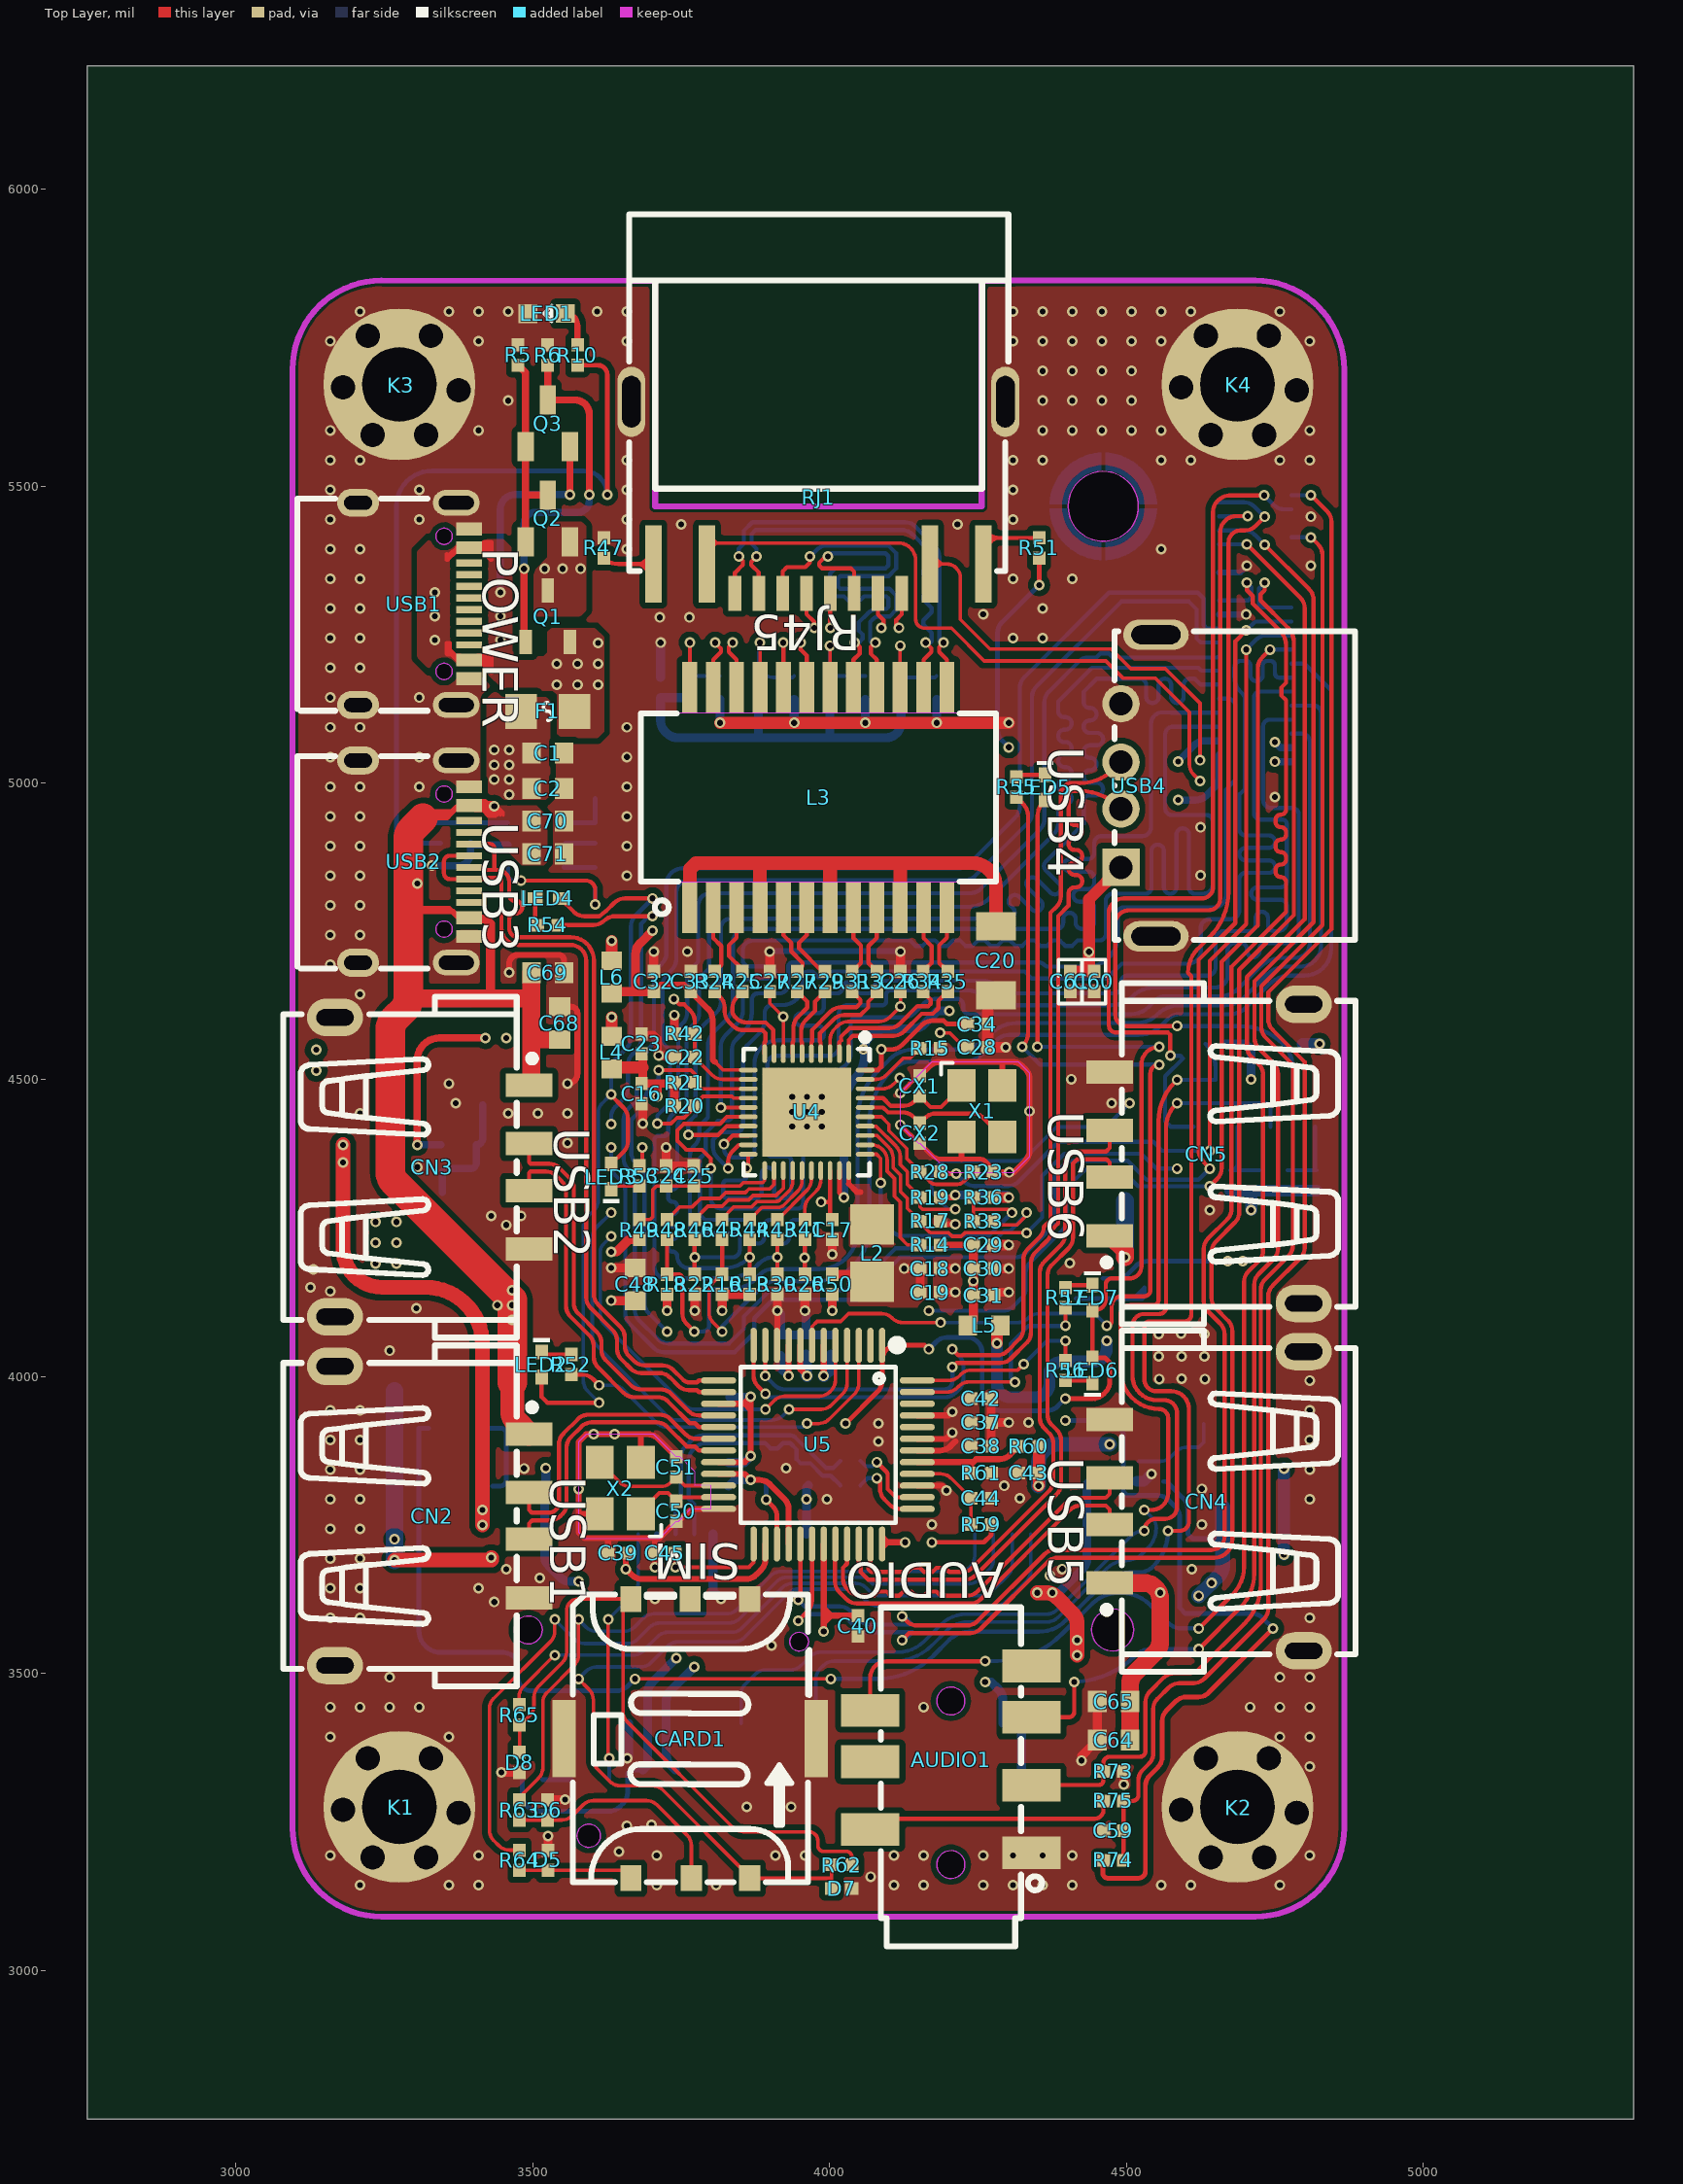
[diagram p0: Top Layer view]
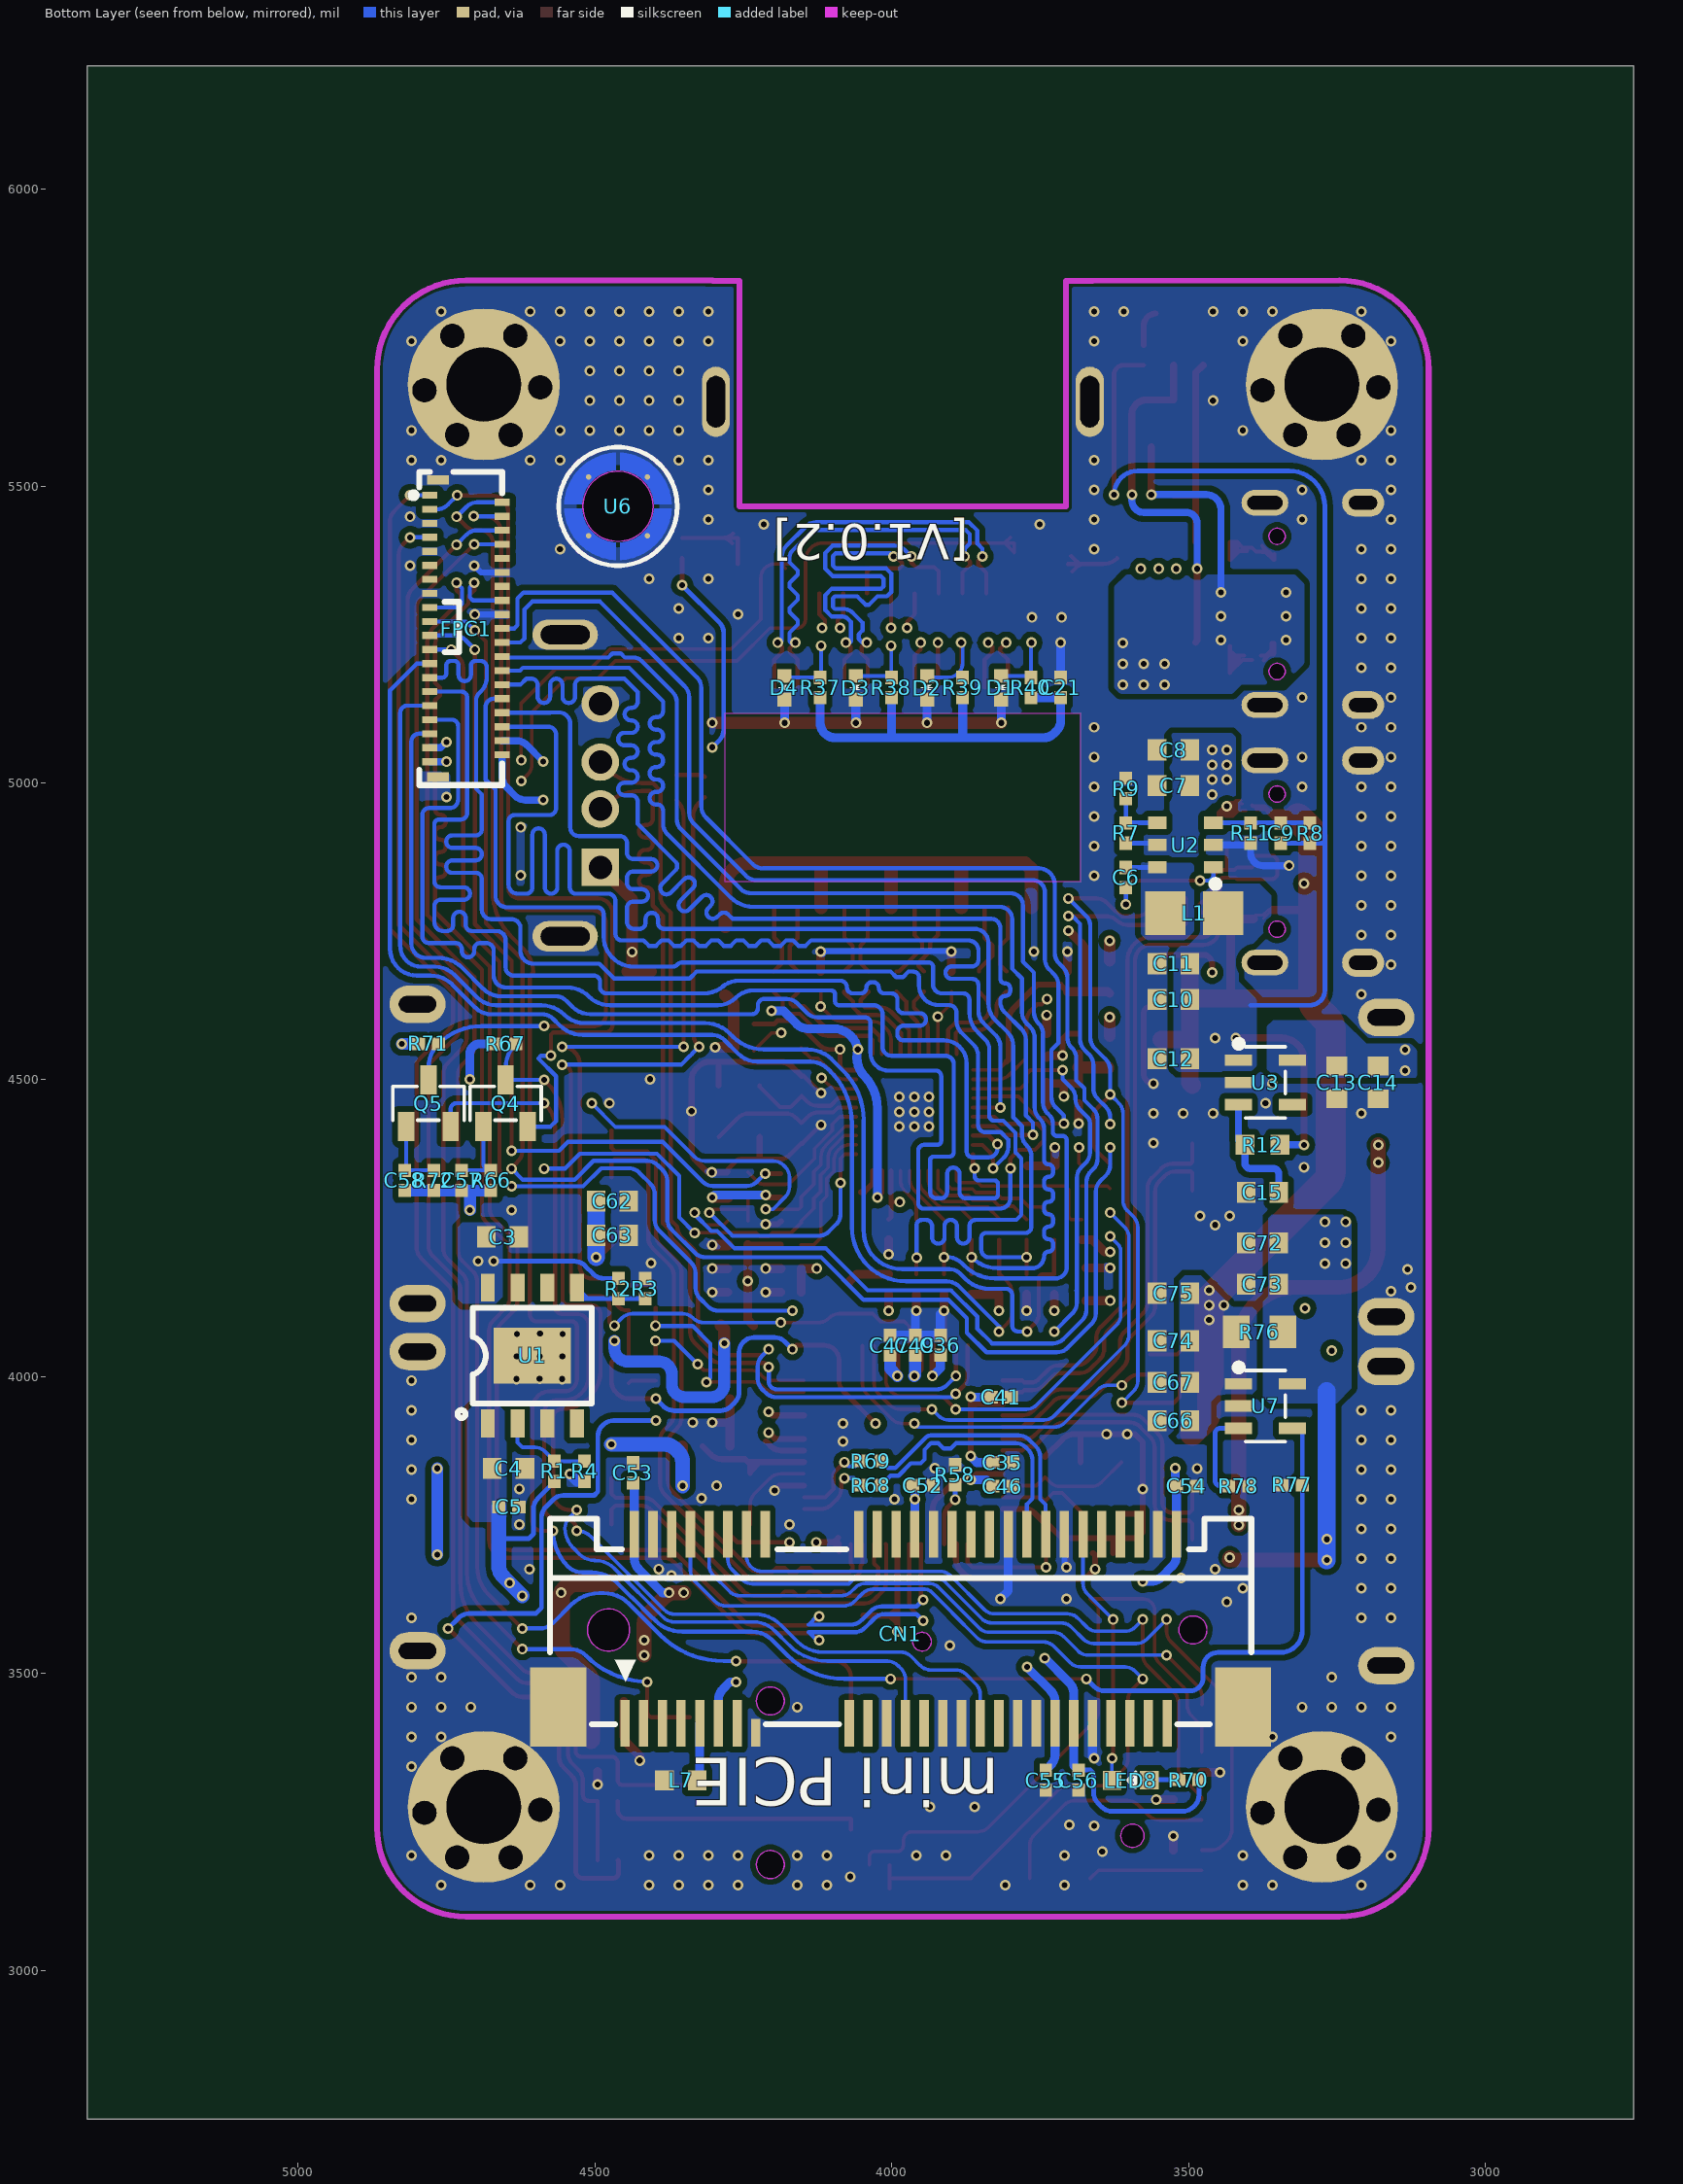
[diagram p1: Bottom Layer view, seen from below]
# Altium PCB MISC84334.PcbDoc (part 1 of 8)
Units mil, origin at the board's own origin, x right, y up, seen from the top; angles counter-clockwise.
Board outline 2605.13 x 3457.4 mil, 4 copper layers (Top Layer, GND, VCC, Bottom Layer), stack 62.447 mil thick; 209 components, 149 nets, 735 pads, 529 vias.

## Layer stack, top to bottom
Top Layer: signal copper 1.378
Dielectric1: surface 8.283, 7628 RC49% 8.6mil, Dk 0
GND: signal copper 0.598
Dielectric2: surface 41.929, 1.1mm H/HOZ 含铜, Dk 0
VCC: signal copper 0.598
Dielectric3: surface 8.283, 7628 RC49% 8.6mil, Dk 0
Bottom Layer: signal copper 1.378

## Board outline
5355.13,2750 2750,2750 2750,6207.4 5355.13,6207.4

## Design rules (kind name [scope] priority, off if disabled: settings)
BoardOutlineClearance copperThickness2oz_1 [All] p2 off: genericclearance=8 ignorepadtopadclearanceinfootprint=FALSE except(0: Arc-SplitContinuation Track-SplitContinuation SMDPad-SplitContinuation THPad-SplitContinuation Via-SplitContinuation Fill-SplitContinuation Region-SplitContinuation Poly-SplitContinuation Text-SplitContinuation Hole-SplitContinuation; 6: Arc-OutlineEdge Track-OutlineEdge SMDPad-OutlineEdge THPad-OutlineEdge Via-OutlineEdge Fill-OutlineEdge Region-OutlineEdge Text-OutlineEdge Hole-OutlineEdge Arc-CutoutEdge Track-CutoutEdge SMDPad-CutoutEdge THPad-CutoutEdge Via-CutoutEdge Fill-CutoutEdge Region-CutoutEdge Text-CutoutEdge Hole-CutoutEdge; 10: Poly-OutlineEdge Poly-CutoutEdge)
BoardOutlineClearance Plane_innerPlane_1 [All] p4 off: genericclearance=4 ignorepadtopadclearanceinfootprint=FALSE except(0: SMDPad-CutoutEdge Arc-SplitContinuation Track-SplitContinuation SMDPad-SplitContinuation THPad-SplitContinuation Via-SplitContinuation Fill-SplitContinuation Region-SplitContinuation Poly-SplitContinuation Text-SplitContinuation Hole-SplitContinuation; 6: Arc-OutlineEdge Track-OutlineEdge SMDPad-OutlineEdge THPad-OutlineEdge Via-OutlineEdge Fill-OutlineEdge Region-OutlineEdge Text-OutlineEdge Hole-OutlineEdge Arc-CutoutEdge Track-CutoutEdge THPad-CutoutEdge Via-CutoutEdge Fill-CutoutEdge Region-CutoutEdge Text-CutoutEdge Hole-CutoutEdge; 10: Poly-OutlineEdge Poly-CutoutEdge)
BoardOutlineClearance Copper_copperRegion_1 [All] p6 off: genericclearance=4 ignorepadtopadclearanceinfootprint=FALSE except(0: SMDPad-CutoutEdge Arc-SplitContinuation Track-SplitContinuation SMDPad-SplitContinuation THPad-SplitContinuation Via-SplitContinuation Fill-SplitContinuation Region-SplitContinuation Poly-SplitContinuation Text-SplitContinuation Hole-SplitContinuation; 6: Arc-OutlineEdge Track-OutlineEdge SMDPad-OutlineEdge THPad-OutlineEdge Via-OutlineEdge Fill-OutlineEdge Region-OutlineEdge Text-OutlineEdge Hole-OutlineEdge Arc-CutoutEdge Track-CutoutEdge THPad-CutoutEdge Via-CutoutEdge Fill-CutoutEdge Region-CutoutEdge Text-CutoutEdge Hole-CutoutEdge; 10: Poly-OutlineEdge Poly-CutoutEdge)
BoardOutlineClearance copperThickness1oz_1 [All] p8: genericclearance=4 ignorepadtopadclearanceinfootprint=FALSE except(0: SMDPad-CutoutEdge Arc-SplitContinuation Track-SplitContinuation SMDPad-SplitContinuation THPad-SplitContinuation Via-SplitContinuation Fill-SplitContinuation Region-SplitContinuation Poly-SplitContinuation Text-SplitContinuation Hole-SplitContinuation; 6: Arc-OutlineEdge Track-OutlineEdge SMDPad-OutlineEdge THPad-OutlineEdge Via-OutlineEdge Fill-OutlineEdge Region-OutlineEdge Text-OutlineEdge Hole-OutlineEdge Arc-CutoutEdge Track-CutoutEdge THPad-CutoutEdge Via-CutoutEdge Fill-CutoutEdge Region-CutoutEdge Text-CutoutEdge Hole-CutoutEdge; 10: Poly-OutlineEdge Poly-CutoutEdge)
Clearance copperThickness2oz [All] p1 off: gap=8 ignorepadtopadclearanceinfootprint=FALSE except(6: SMDPad-Track SMDPad-SMDPad THPad-Track SMDPad-THPad THPad-THPad Track-Via SMDPad-Via THPad-Via Via-Via Fill-Track Region-Track Fill-SMDPad Region-SMDPad Fill-THPad Region-THPad Fill-Via Region-Via Fill-Fill Fill-Region Region-Region Arc-SMDPad Arc-THPad Arc-Via Fill-Arc Region-Arc Arc-Arc Text-Track SMDPad-Text Text-THPad Text-Via Fill-Text Region-Text Text-Text Hole-Track Hole-SMDPad Hole-THPad Hole-Via Fill-Hole Region-Hole Hole-Arc Hole-Text; 10: Poly-Track Poly-SMDPad Poly-THPad Poly-Via Poly-Fill Poly-Region Poly-Poly Poly-Arc Poly-Text Poly-Hole; 11.8: Arc-Track Arc-Text)
Clearance Plane_innerPlane [All] p3 off: gap=4 ignorepadtopadclearanceinfootprint=FALSE except(6: SMDPad-Track SMDPad-SMDPad THPad-Track SMDPad-THPad THPad-THPad Track-Via SMDPad-Via THPad-Via Via-Via Fill-Track Region-Track Fill-SMDPad Region-SMDPad Fill-THPad Region-THPad Fill-Via Region-Via Fill-Fill Fill-Region Region-Region Arc-SMDPad Arc-THPad Arc-Via Fill-Arc Region-Arc Arc-Arc Text-Track SMDPad-Text Text-THPad Text-Via Fill-Text Region-Text Text-Text Hole-Track Hole-SMDPad Hole-THPad Hole-Via Fill-Hole Region-Hole Hole-Arc Hole-Text; 10: Poly-Track Poly-SMDPad Poly-THPad Poly-Via Poly-Fill Poly-Region Poly-Poly Poly-Arc Poly-Text Poly-Hole; 11.8: Arc-Track Arc-Text)
Clearance Copper_copperRegion [All] p5 off: gap=4 ignorepadtopadclearanceinfootprint=FALSE except(6: SMDPad-Track SMDPad-SMDPad THPad-Track SMDPad-THPad THPad-THPad Track-Via SMDPad-Via THPad-Via Via-Via Fill-Track Region-Track Fill-SMDPad Region-SMDPad Fill-THPad Region-THPad Fill-Via Region-Via Fill-Fill Fill-Region Region-Region Arc-SMDPad Arc-THPad Arc-Via Fill-Arc Region-Arc Arc-Arc Text-Track SMDPad-Text Text-THPad Text-Via Fill-Text Region-Text Text-Text Hole-Track Hole-SMDPad Hole-THPad Hole-Via Fill-Hole Region-Hole Hole-Arc Hole-Text; 10: Poly-Track Poly-SMDPad Poly-THPad Poly-Via Poly-Fill Poly-Region Poly-Poly Poly-Arc Poly-Text Poly-Hole; 11.8: Arc-Track Arc-Text)
Clearance copperThickness1oz [All] p7: gap=4 ignorepadtopadclearanceinfootprint=FALSE except(6: SMDPad-Track SMDPad-SMDPad THPad-Track SMDPad-THPad THPad-THPad Track-Via SMDPad-Via THPad-Via Via-Via Fill-Track Region-Track Fill-SMDPad Region-SMDPad Fill-THPad Region-THPad Fill-Via Region-Via Fill-Fill Fill-Region Region-Region Arc-SMDPad Arc-THPad Arc-Via Fill-Arc Region-Arc Arc-Arc Text-Track SMDPad-Text Text-THPad Text-Via Fill-Text Region-Text Text-Text Hole-Track Hole-SMDPad Hole-THPad Hole-Via Fill-Hole Region-Hole Hole-Arc Hole-Text; 10: Poly-Track Poly-SMDPad Poly-THPad Poly-Via Poly-Fill Poly-Region Poly-Poly Poly-Arc Poly-Text Poly-Hole; 11.8: Arc-Track Arc-Text)
DiffPairsRouting differentialPair [All] p1: maxlimit=6 minlimit=6 mostfreqgap=6 toplayer_minwidth=7 toplayer_prefwidth=7 toplayer_maxwidth=7 toplayer_mingap=6 toplayer_prefgap=6 toplayer_maxgap=6 midlayer1_minwidth=7 midlayer1_prefwidth=7 midlayer1_maxwidth=7 midlayer1_mingap=6 midlayer1_prefgap=6 midlayer1_maxgap=6 midlayer2_minwidth=7 midlayer2_prefwidth=7 midlayer2_maxwidth=7 midlayer2_mingap=6 midlayer2_prefgap=6 midlayer2_maxgap=6 bottomlayer_minwidth=7 bottomlayer_prefwidth=7 bottomlayer_maxwidth=7 bottomlayer_mingap=6 bottomlayer_prefgap=6 bottomlayer_maxgap=6 maxuncoupledlength=10
HoleToHoleClearance otherClearance [All] p1: gap=11.8 allowstackedmicrovias=TRUE
Length netLength [All] p1: minlimit=0 maxlimit=0
PasteMaskExpansion pasteMaskExpansion [All] p1: expansion=0
PlaneConnect innerPlane [All] p1: planeconnectstyle=Relief reliefexpansion=20 reliefentries=4 reliefconductorwidth=10 reliefairgap=10
PolygonConnect copperRegion [All] p1: connectstyle=Direct reliefconductorwidth=10 reliefentries=4 polygonreliefangle="90 Angle" airgapwidth=10 via.connectstyle=Relief via.reliefconductorwidth=10 via.reliefentries=4 via.polygonreliefangle="90 Angle" via.airgapwidth=10
RoutingVias viaSize [All] p1: holewidth=10 width=18 viastyle="Through Hole" minholewidth=10 minwidth=18 maxholewidth=10 maxwidth=18
SolderMaskExpansion solderMaskExpansion [IsVia] p1: expansion=-1000 istentingtop=TRUE
SolderMaskExpansion solderMaskExpansion [All] p2: expansion=2 istentingtop=FALSE
Width copperThickness2oz_2 [All] p1 off: maxlimit=100 minlimit=8 preferedwidth=10
Width copperThickness1oz_2 [All] p2: maxlimit=100 minlimit=5 preferedwidth=7

## Components (designator, comment, footprint, x,y, rotation, side; value= is the part's Value field where it differs from the comment)
AUDIO1 "PJ-393" AUDIO-SMD_PJ-393 4204.62,3355.59 r0 top
C1 "10uF" r0603#1 3525.59,5050.59 r180 top
C2 "100nF" r0603#1 3525.59,4990.59 r180 top
C3 "4.7uF" C0603 4655.59,4235.59 r0 bottom
C4 "4.7uF" C0603 4645.59,3845.59 r0 bottom
C5 "100nF" R0402 4645.29,3780.59 r0 bottom
C6 "100nF" R0402 3605.59,4840.59 r270 bottom
C7 "10uF" r0603#2 3525.59,4995.59 r180 bottom
C8 "100nF" r0603#2 3525.59,5055.59 r180 bottom
C9 "22pF" R0402 3344.86,4915.59 r270 bottom
C10 "22uF" r0603#2 3525.59,4635.59 r180 bottom
C11 "100nF" r0603#2 3525.59,4695.59 r180 bottom
C12 "10uF" r0603#1 3525.59,4535.59 r180 bottom
C13 "4.7uF" r0603#1 3250.59,4495.59 r90 bottom
C14 "100nF" C0603 3180.59,4495.59 r90 bottom
C15 "100nF" C0603 3375.59,4310.59 r180 bottom
C16 "100nF" R0402 3683.59,4476.71 r90 top
C17 "100nF" R0402 4005.09,4247.85 r90 top
C18 "100nF" R0402 4169.59,4182.09 r180 top
C19 "4.7uF" R0402 4169.83,4142.09 r180 top
C20 "10nF" r1206 4280.59,4700.59 r90 top
C21 "1nF" R0402 3715.59,5160.59 r270 bottom
C22 "100nF" R0402 3756.09,4538.09 r0 top
C23 "100nF" R0402 3683.59,4560.59 r270 top
C24 "100nF" R0402 3725.09,4338.09 r270 top
C25 "100nF" R0402 3771.52,4338.09 r270 top
C26 "100nF" R0402 4119.79,4665.59 r270 top
C27 "100nF" R0402 3899.65,4665.59 r270 top
C28 "100nF" R0402 4249.48,4555.09 r180 top
C29 "100nF" R0402 4259.59,4222.09 r180 top
C30 "100nF" R0402 4259.59,4182.09 r180 top
C31 "100nF" R0402 4259.59,4137.09 r180 top
C32 "100nF" R0402 3704.09,4665.59 r270 top
C33 "100nF" R0402 3766.55,4665.59 r270 top
C34 "100nF" R0402 4249.48,4594.09 r180 top
C35 "100nF" R0402 3813.09,3855.59 r0 bottom
C36 "100nF" R0402 3918.09,4053.09 r270 bottom
C37 "100nF" R0402 4255.6,3923.09 r180 top
C38 "100nF" R0402 4255.6,3883.09 r180 top
C39 "100nF" R0402 3644.19,3703.09 r0 top
C40 "100nF" R0402 4048.09,3580.59 r90 top
C41 "100nF" R0402 3815.59,3965.59 r0 bottom
C42 "100nF" R0402 4255.6,3963.09 r180 top
C43 "100nF" R0402 4335.95,3838.09 r0 top
C44 "100nF" R0402 4255.6,3795.59 r180 top
C45 "100nF" R0402 3723.14,3703.09 r0 top
C46 "100nF" R0402 3813.09,3815.59 r0 bottom
C47 "100nF" R0402 4003.09,4053.09 r270 bottom
C48 "10uF" r0603#1 3673,4155.59 r270 top
C49 "100nF" R0402 3960.59,4053.09 r270 bottom
C50 "12pF" R0402 3742.02,3773.39 r90 top
C51 "12pF" R0402 3742.02,3848.09 r90 top
C52 "100nF" R0402 3947.55,3817.03 r0 bottom
C53 "100nF" R0402 4436.02,3838.07 r270 bottom
C54 "100nF" R0402 3503.47,3816.03 r0 bottom
C55 "100nF" R0402 3740.59,3320.59 r90 bottom
C56 "100nF" R0402 3685.59,3320.59 r90 bottom
C57 "1nF" r0402 4724.41,4330.59 r90 bottom
C58 "1nF" r0402 4820.59,4330.59 r270 bottom
C59 "100nF" R0402 4478.65,3235.59 r180 top
C60 "100nF" R0402 4445.59,4665.59 r90 top
C61 "10uF" R0402 4405.59,4665.59 r90 top
C62 "100nF" r0603#1 4470.59,4295.59 r0 bottom
C63 "10uF" r0603#1 4470.59,4238.09 r0 bottom
C64 "100nF" r0603#1 4478.96,3388.09 r0 top
C65 "10uF" r0603#1 4478.96,3453.09 r0 top
C66 "100nF" r0603#1 3525.59,3925.59 r180 bottom
C67 "10uF" r0603#1 3525.59,3990.59 r180 bottom
C68 "100nF" r0603#1 3545.59,4595.59 r270 top
C69 "10uF" r0603#1 3525.59,4680.59 r180 top
C70 "100nF" r0603#1 3525.59,4935.59 r180 top
C71 "10uF" r0603#1 3525.59,4880.59 r180 top
C72 "100nF" C0603 3375.59,4225.59 r0 bottom
C73 "1uF" C0603 3375.59,4155.59 r180 bottom
C74 "100nF" C0603 3525.59,4060.59 r180 bottom
C75 "10uF" C0603 3525.59,4140.59 r180 bottom
CARD1 "SMN-304" SIM-SMD_SMN-304 3765.59,3390.59 r0 top locked
CN1 "1775862-2" PCI-SMD_1775862-2 3984.96,3575.59 r0 bottom locked
CN2 "908-161A2021S10110" USB-A-SMD_AF-SMT-SHORT 3330.59,3765.59 r270 top locked
CN3 "908-161A2021S10110" USB-A-SMD_AF-SMT-SHORT 3330.59,4353.09 r270 top locked
CN4 "908-161A2021S10110" USB-A-SMD_AF-SMT-SHORT 4635.59,3790.38 r90 top locked
CN5 "908-161A2021S10110" USB-A-SMD_AF-SMT-SHORT 4635.59,4375.38 r90 top
CX1 "12pF" R0402 4152.05,4489.59 r270 top
CX2 "12pF" R0402 4152.35,4410.09 r90 top
D1 "KLXES15AAA1" D0402-BI 3815.59,5160.43 r270 bottom
D2 "KLXES15AAA1" D0402-BI 3940.59,5160.43 r270 bottom
D3 "KLXES15AAA1" D0402-BI 4060.59,5160.43 r270 bottom
D4 "KLXES15AAA1" D0402-BI 4180.59,5160.43 r270 bottom
D5 "KLXES15AAA1" R0402 3525.8,3185.59 r90 top
D6 "KLXES15AAA1" R0402 3525.59,3270.59 r90 top
D7 "KLXES15AAA1" R0402 4020.59,3138.09 r0 top
D8 "KLXES15AAA1" R0402 3478.04,3350.59 r270 top
F1 "BSMD0805L-200" F0805 3525.59,5120.59 r180 top
FPC1 "AFE03-S39FMA-1H" fpc-smd_p0.30-39p_fgs-xj-h1.0 4717.29,5260.09 r270 bottom
K1 "" "125 X 300" 3275.59,3275.59 r0 top
K2 "" "125 X 300" 4687.29,3275.59 r0 top
K3 "" "125 X 300" 3275.59,5671.19 r0 top locked
K4 "" "125 X 300" 4687.29,5671.19 r0 top locked
L1 "2.2uH" IND-SMD_L2.5-W2.0_WPN252012H 3490.59,4780.59 r0 bottom
L2 "2.2uH" IND-SMD_L2.5-W2.0_WPN252012H 4071.95,4208.09 r90 top
L3 "G2406S" SMD-24_L15.1-W7.1-P1.00-LS10.0-BL 3981.44,4975.59 r0 top locked
L4 "CBM160808U121T" L0603 3633.09,4545.86 r90 top
L5 "CBM160808U121T" L0603 4260.56,4086.09 r0 top
L6 "CBM160808U121T" L0603 3633.09,4673.09 r90 top
L7 "CBG160808U000T" L0603 4355.59,3320.23 r180 bottom
LED1 "19-217/GHC-YR1S2/3T" LED0603-RD 3525.59,5790.59 r0 top